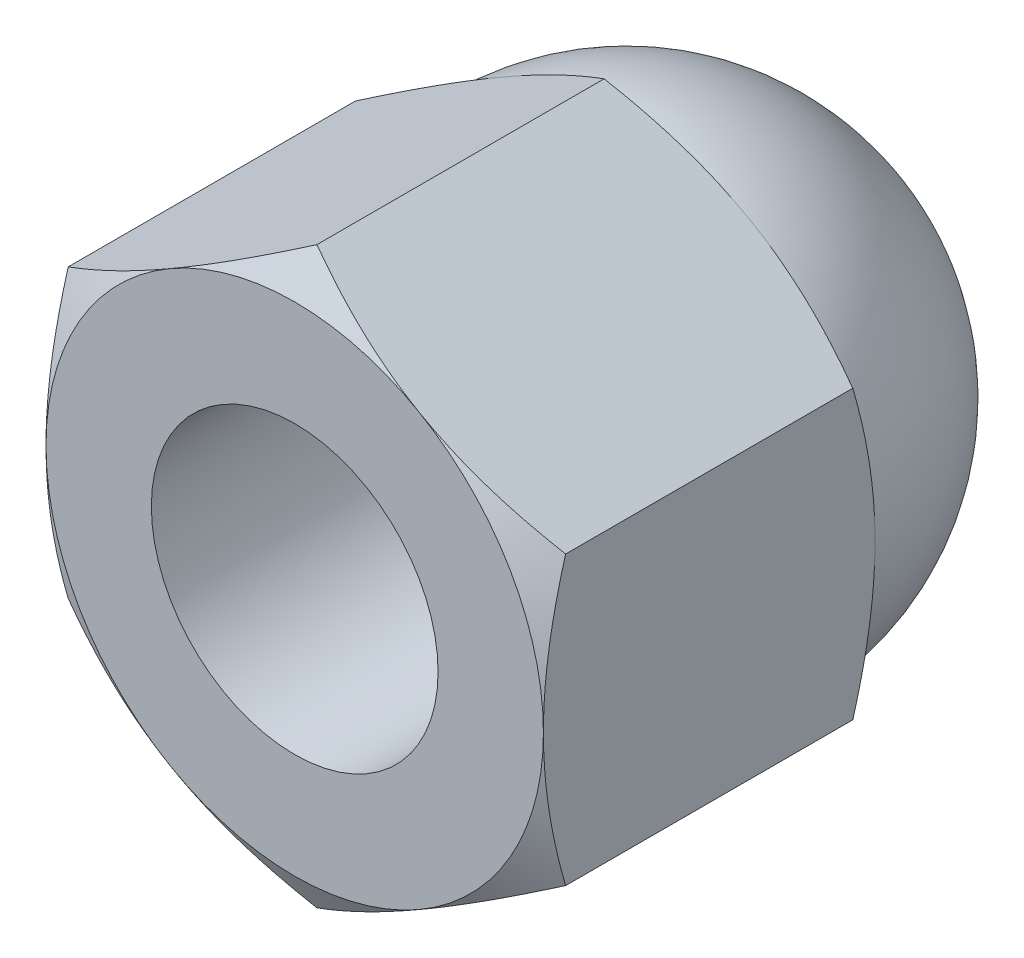
SolidWorks part; units mm, degrees
ref_plane "前视" through (0, 0, 0) normal (0, 0, 1) x (1, 0, 0)
ref_plane "上视" through (0, 0, 0) normal (0, 1, 0) x (1, 0, 0)
ref_plane "右视" through (0, 0, 0) normal (1, 0, 0) x (0, 0, -1)
sketch "尺寸草图" plane through (0, 0, 0) normal (1, 0, 0) x (0, 0, -1)
  line L0 (0, 20.03) -> (0, 0)
  line L1 (0, 0) -> (-12, 0)
  line L2 (-12, 0) -> (-12, 1.5)
  line L3 (-12, 1.5) -> (-12, 23.1)
  line L4 (-12, 23.1) -> (-12, 35.1)
  line L5 (-12, 35.1) -> (6, 35.1)
  line L6 (6, 35.1) -> (22.6, 35.1)
  line L7 (22.6, 35.1) -> (22.6, 25.5)
  line L8 (22.6, 25.5) -> (22.6, 7.77)
  point P4 (0, 12)
  point P6 (-22, 0)
  point P7 (-2, 0)
  point P8 (0, 9)
  point P9 (-18, 0)
  dimension "m" = 12
  dimension "e" = 20.03
  dimension "d" = 12
  dimension "h" = 22
  dimension "b" = 10
  dimension "R" = 9
  dimension "s" = 18
  dimension "P" = 1.5
  dimension "da(max)" = 21.6
  dimension "da(min)" = 12
  dimension "dk" = 18
  dimension "dw" = 16.6
  dimension "mw" = 9.6
  dimension "s(min)" = 17.73
sketch "草图1" plane through (0, 0, 0) normal (0, 0, 1) x (1, 0, 0)
  line L1 (0, 10.3923) -> (-9, 5.1962)
  line L2 (-9, 5.1962) -> (-9, -5.1962)
  line L3 (-9, -5.1962) -> (0, -10.3923)
  line L4 (0, -10.3923) -> (9, -5.1962)
  line L5 (9, -5.1962) -> (9, 5.1962)
  line L6 (9, 5.1962) -> (0, 10.3923)
  circle A0 centre (0, 0) radius 9 construction
  dimension "D1" = 18
extrude "基体-拉伸" add sketch "草图1" along normal blind 12
sketch "草图2" plane through (0, 0, 0) normal (0, 1, 0) x (1, 0, 0)
  line L0 (0, 2.5796) -> (0, -0.4985) construction
  line L1 (0, 9) -> (0, 0)
  line L2 (9, 0) -> (0, 0)
  arc A0 (9, 0) -> (0, 9) centre (0, 0) ccw
  dimension "D1" = 9
revolve "凸台-旋转1" add sketch "草图2" angle 360 about L0
sketch "草图4" plane through (0, 0, 0) normal (0, 0, -1) x (-1, 0, 0)
  circle A0 centre (0, 0) radius 9
  circle A1 centre (0, 0) radius 9 construction
extrude "切除-拉伸1" cut sketch "草图4" against normal through all draft 60 flip side to cut
sketch "草图5" plane through (0, 0, 12) normal (0, 0, 1) x (1, 0, 0)
  circle A0 centre (0, 0) radius 9
  circle A1 centre (0, 0) radius 9 construction
extrude "切除-拉伸2" cut sketch "草图5" against normal through all draft 60 flip side to cut
sketch "草图6" plane through (0, 0, 12) normal (0, 0, 1) x (1, 0, 0)
  circle A0 centre (0, 0) radius 5.1881
  dimension "D1" = 10.3763
extrude "切除-拉伸3" cut sketch "草图6" against normal blind 10
cosmetic thread "装饰螺纹线1" parameters "D2"=12
